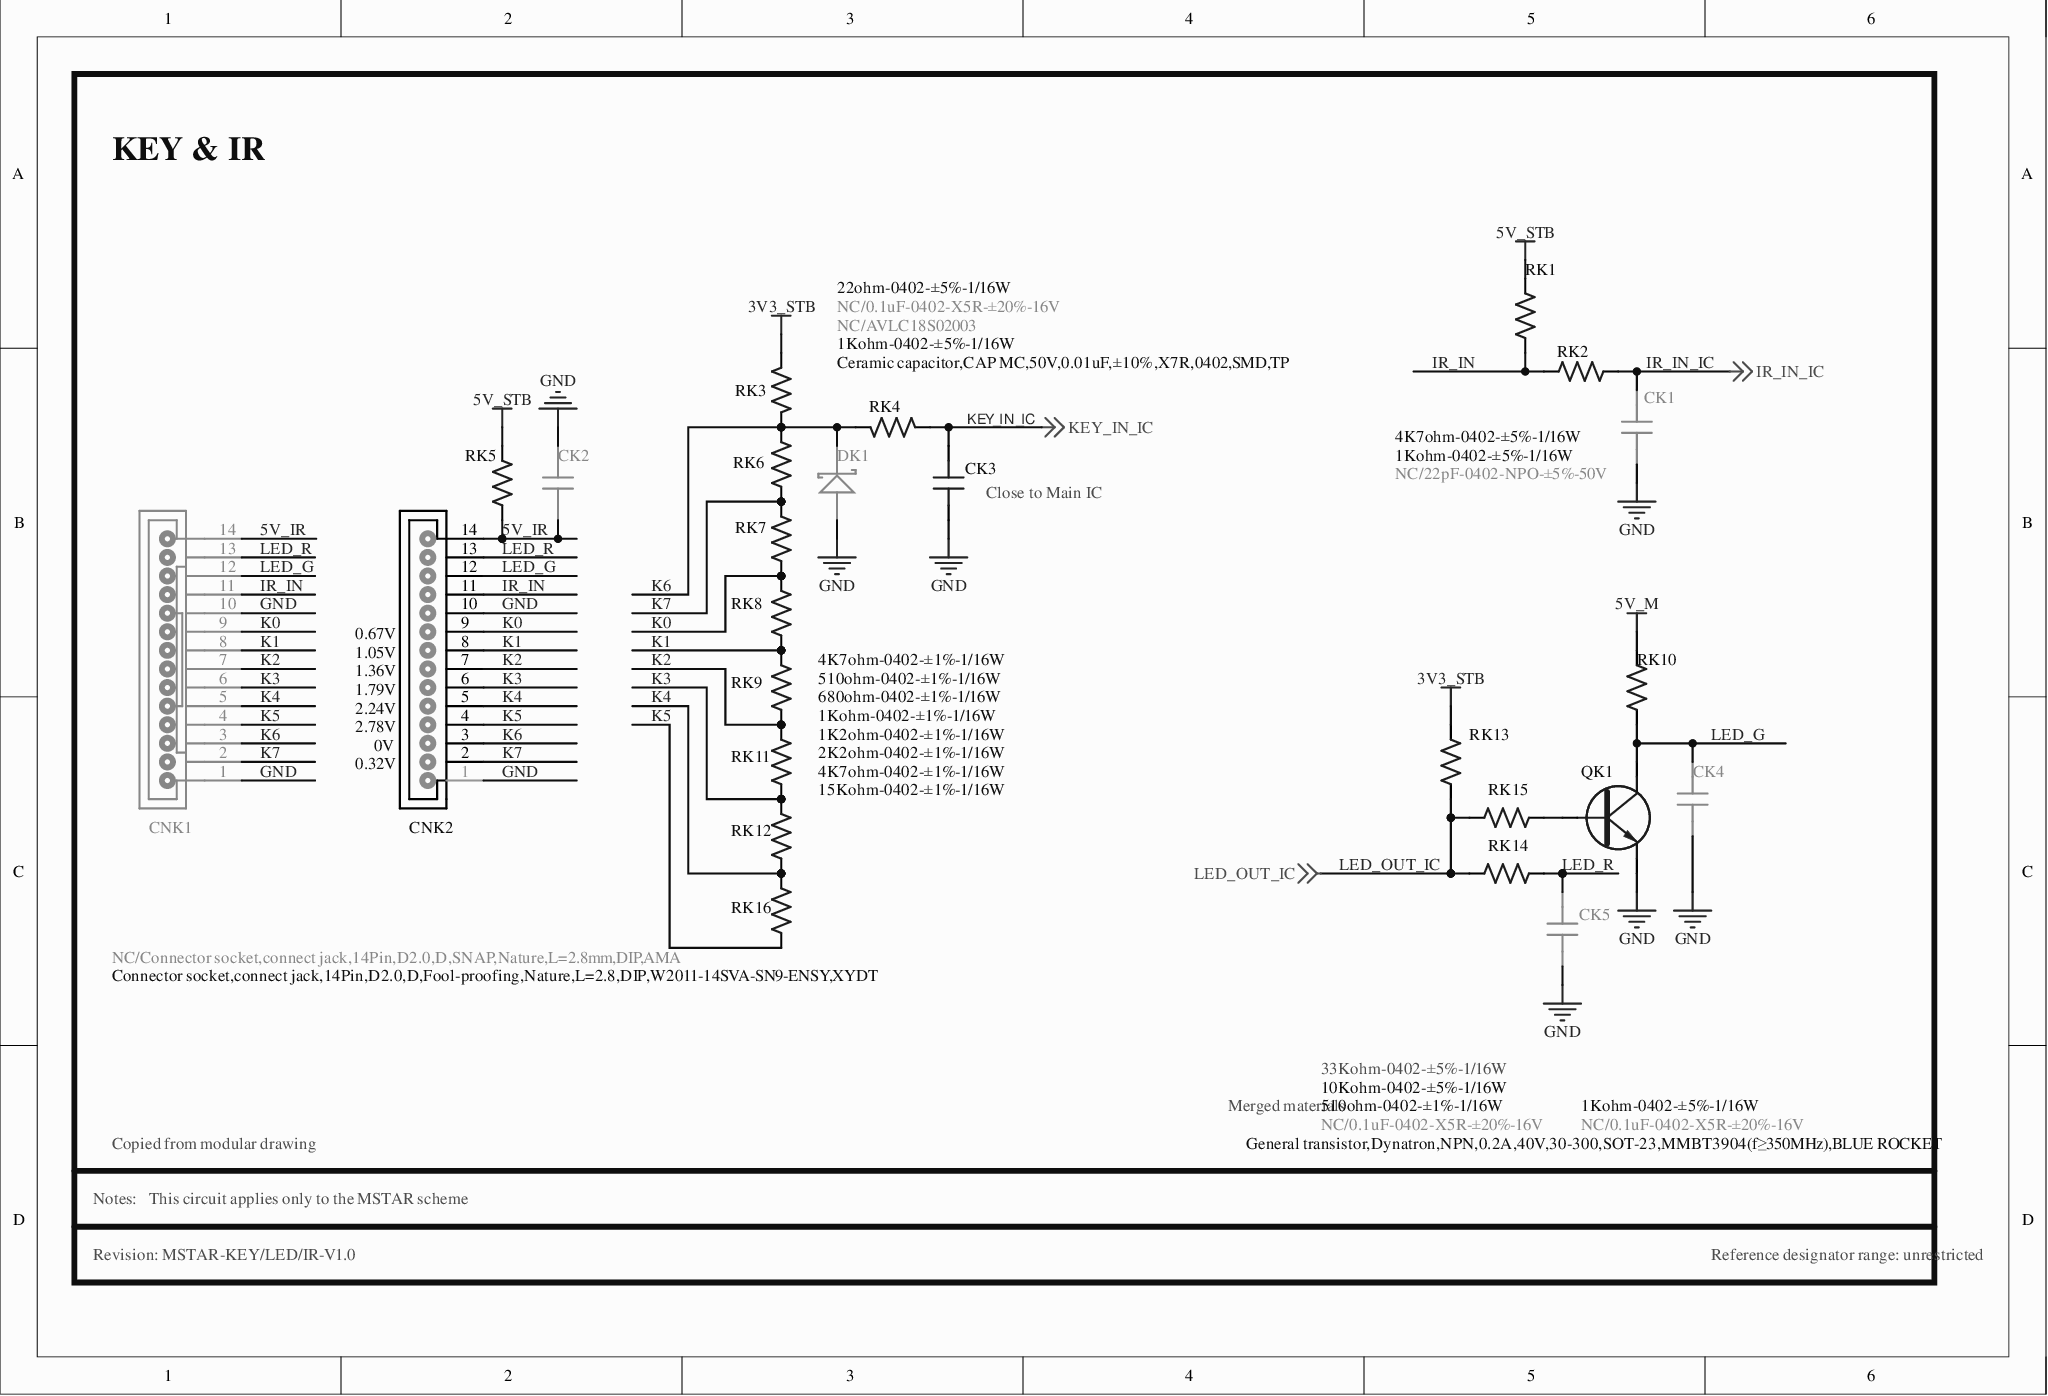
[diagram p0: MISC86372-10.SchDoc]
# Altium project MISC86372-32.PrjPCB (part 4 of 8)

## Sheet MISC86372-10.SchDoc
size 279 x 190 mm

### Parts
CK1  NC/22pF-0402-NPO-±5%-50V  [C0402]
CK2  NC/0.1uF-0402-X5R-±20%-16V  [C0402]
CK3  Ceramic capacitor,CAP MC,50V,0.01uF,±10%,X7R,0402,SMD,TP  [C0402]
CK4  NC/0.1uF-0402-X5R-±20%-16V  [C0402]
CK5  NC/0.1uF-0402-X5R-±20%-16V  [C0402]
CNK1  NC/Connector socket,connect jack,14Pin,D2.0,D,SNAP,Nature,L=2.8mm,DIP,AMA  [SIP14/2.0D-5]
CNK2  Connector socket,connect jack,14Pin,D2.0,D,Fool-proofing,Nature,L=2.8,DIP,W2011-14SVA-SN9-ENSY,XYDT  [SIP14/2.0D-1]
DK1  NC/AVLC18S02003  [DIODE-S0402]
QK1  General transistor,Dynatron,NPN,0.2A,40V,30-300,SOT-23,MMBT3904(f≥350MHz),BLUE ROCKET  [SOT-23]
RK1  4K7ohm-0402-±5%-1/16W  [R0402]
RK2  1Kohm-0402-±5%-1/16W  [R0402]
RK3  4K7ohm-0402-±1%-1/16W  [R0402]
RK4  1Kohm-0402-±5%-1/16W  [R0402]
RK5  22ohm-0402-±5%-1/16W  [R0402]
RK6  510ohm-0402-±1%-1/16W  [R0402]
RK7  680ohm-0402-±1%-1/16W  [R0402]
RK8  1Kohm-0402-±1%-1/16W  [R0402]
RK9  1K2ohm-0402-±1%-1/16W  [R0402]
RK10  1Kohm-0402-±5%-1/16W  [R0402]
RK11  2K2ohm-0402-±1%-1/16W  [R0402]
RK12  4K7ohm-0402-±1%-1/16W  [R0402]
RK13  33Kohm-0402-±5%-1/16W  [R0402]
RK14  510ohm-0402-±1%-1/16W  [R0402]
RK15  10Kohm-0402-±5%-1/16W  [R0402]
RK16  15Kohm-0402-±1%-1/16W  [R0402]

### Nets
3V3_STB: RK3.2 RK13.2
5V_M: RK10.2
5V_STB: RK1.2 RK5.1
GND: CK1.1 CK2.1 CK3.1 CK4.2 CK5.2 CNK1.1 CNK1.10 CNK2.1 CNK2.10 DK1.A QK1.E
5V_IR: CK2.2 CNK1.14 CNK2.14 RK5.2
IR_IN: CNK1.11 CNK2.11 RK1.1 RK2.1
IR_IN_IC: CK1.2 RK2.2 ; off-sheet IR_IN_IC
K0: CNK1.9 CNK2.9 RK7.1 RK8.2
K1: CNK1.8 CNK2.8 RK8.1 RK9.2
K2: CNK1.7 CNK2.7 RK9.1 RK11.2
K3: CNK1.6 CNK2.6 RK11.1 RK12.2
K4: CNK1.5 CNK2.5 RK12.1 RK16.2
K5: CNK1.4 CNK2.4 RK16.1
K6: CNK1.3 CNK2.3 DK1.K RK3.1 RK4.2 RK6.2
K7: CNK1.2 CNK2.2 RK6.1 RK7.2
KEY_IN_IC: CK3.2 RK4.1 ; off-sheet KEY_IN_IC
LED_G: CK4.1 CNK1.12 CNK2.12 QK1.C RK10.1
LED_OUT_IC: RK13.1 RK14.2 RK15.2 ; off-sheet LED_OUT_IC
LED_R: CK5.1 CNK1.13 CNK2.13 RK14.1
NetQK1_B: QK1.B RK15.1

### Notes on the sheet
- KEY & IR
- (near CK3) Close to Main IC
- (near CNK2) 0.67V
- (near CNK2) 1.05V
- (near CNK2) 1.36V
- (near CNK2) 1.79V
- (near CNK2) 2.24V
- (near CNK2) 2.78V
- (near CNK2) 0.32V
- (near CNK2) 0V
- Copied from modular drawing
- Merged materials
- Notes:
- This circuit applies only to the MSTAR scheme
- Revision: MSTAR-KEY/LED/IR-V1.0
- Reference designator range: unrestricted

### Library data of the parts
CK1 = 22pF-0402-NPO-±5%-50V-D
CK2 CK4 CK5 = 0.1uF-0402-X5R-±20%-16V-D
CK3 = 004.003.0000506-D: Ceramic capacitor,CAP MC,50V,0.01uF,±10%,X7R,0402,SMD,TP-D
CNK1 = 14PIN-2.0-D-H-G-带扣-J-DHMI
CNK2 = 14PIN-2.0-D-H-G-DHMI
DK1 = AVLC18S02003-D
QK1 = LMBT3904LT1G-D-NPN: Q-NPN-#-#-#
RK1 = 4K7ohm-0402-±5%-1/16W-D
RK2 RK4 RK10 = 1Kohm-0402-±5%-1/16W-D
RK3 RK12 = 4K7ohm-0402-±1%-1/16W-D
RK5 = 22ohm-0402-±5%-1/16W-D
RK6 RK14 = 510ohm-0402-±5%-1/16W-D
RK7 = 680ohm-0402-±1%-1/16W-D
RK8 = 1Kohm-0402-±1%-1/16W-D
RK9 = 1K2ohm-0402-±1%-1/16W-D
RK11 = 2K2ohm-0402-±1%-1/16W-D
RK13 = 33Kohm-0402-±5%-1/16W-D
RK15 = 10Kohm-0402-±5%-1/16W-D
RK16 = 15Kohm-0402-±1%-1/16W-D

## Sheet MISC86372-11.SchDoc
size 215 x 228 mm
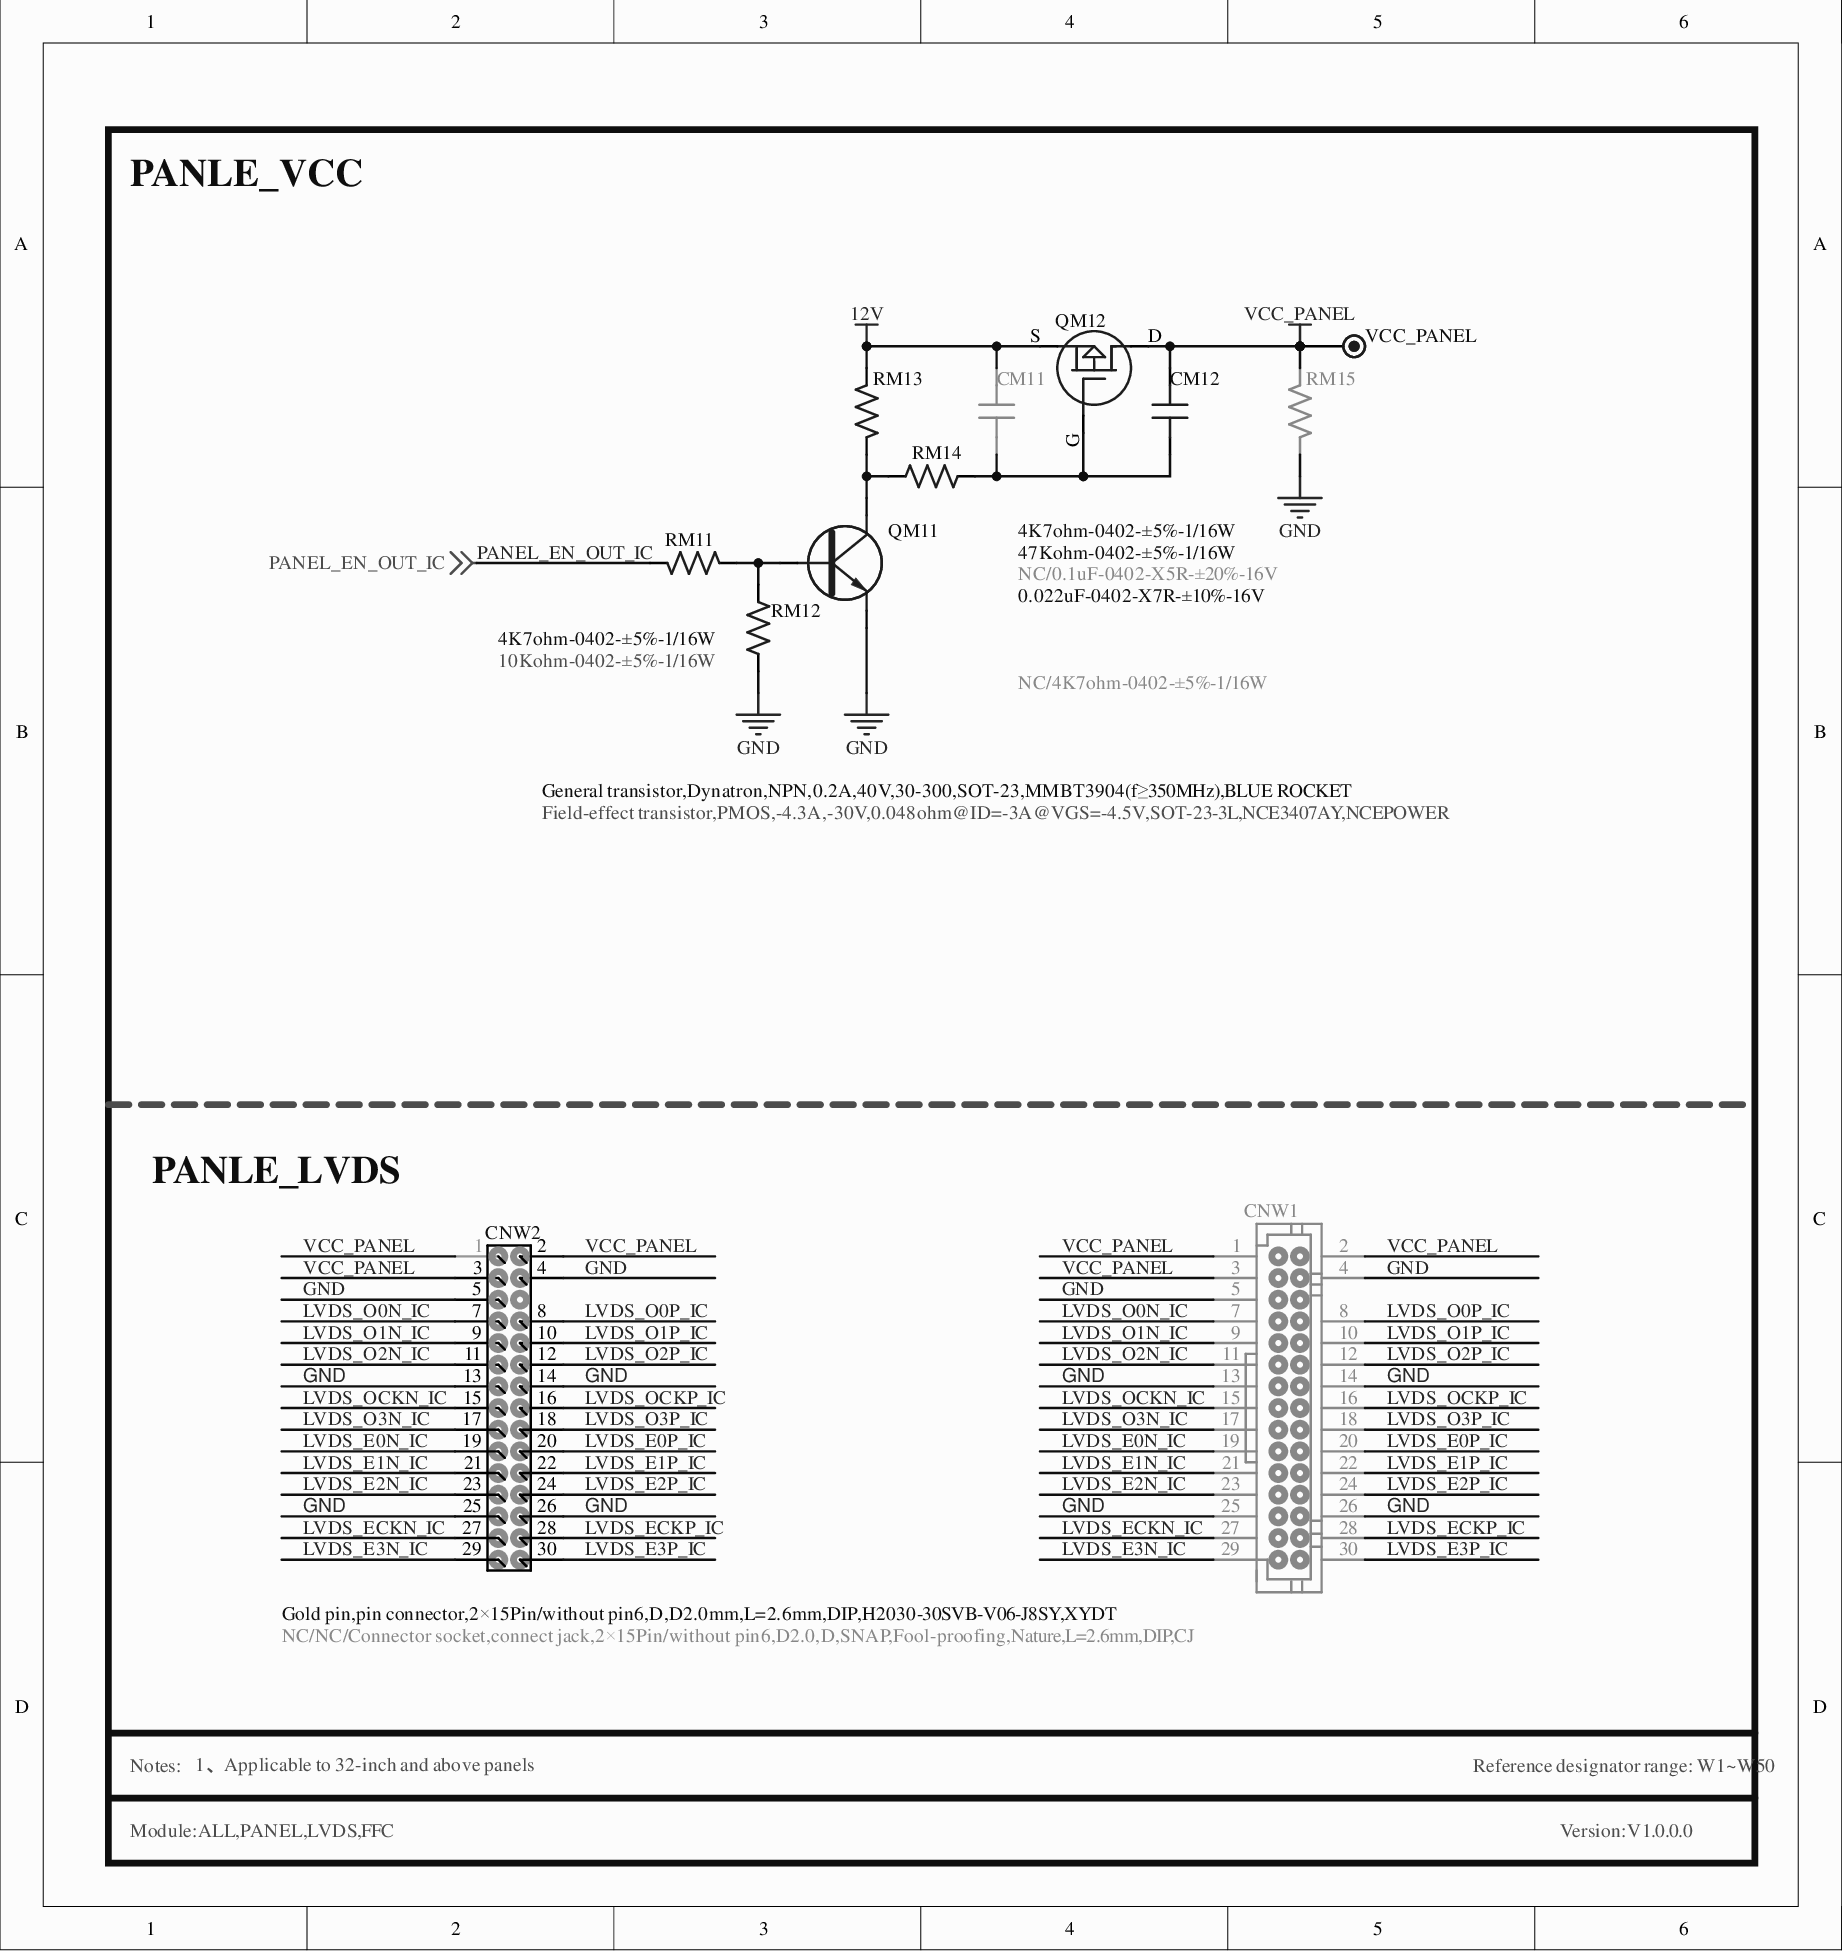
[diagram p1: MISC86372-11.SchDoc]

### Parts
CM11  NC/0.1uF-0402-X5R-±20%-16V  [C0402]
CM12  0.022uF-0402-X7R-±10%-16V  [C0402]
CNW1  NC/NC/Connector socket,connect jack,2×15Pin/without pin6,D2.0,D,SNAP,Fool-proofing,Nature,L=2.6mm,DIP,CJ  [SIP2*15/2.0D-11]
CNW2  Gold pin,pin connector,2×15Pin/without pin6,D,D2.0mm,L=2.6mm,DIP,H2030-30SVB-V06-J8SY,XYDT  [SIP2*15/2.0D-2]
QM11  General transistor,Dynatron,NPN,0.2A,40V,30-300,SOT-23,MMBT3904(f≥350MHz),BLUE ROCKET  [SOT-23]
QM12  Field-effect transistor,PMOS,-4.3A,-30V,0.048ohm@ID=-3A@VGS=-4.5V,SOT-23-3L,NCE3407AY,NCEPOWER  [SOT-23-1]
RM11  4K7ohm-0402-±5%-1/16W  [R0402]
RM12  10Kohm-0402-±5%-1/16W  [R0402]
RM13  4K7ohm-0402-±5%-1/16W  [R0402]
RM14  47Kohm-0402-±5%-1/16W  [R0402]
RM15  NC/4K7ohm-0402-±5%-1/16W  [R0402]
VCC_PANEL  TEST  [TP]  (value not drawn)

### Nets
12V: CM11.2 QM12.S RM13.1
GND: CNW1.4 CNW1.5 CNW1.13 CNW1.14 CNW1.25 CNW1.26 CNW2.4 CNW2.5 CNW2.13 CNW2.14 CNW2.25 CNW2.26 QM11.E RM12.2 RM15.2
VCC_PANEL: CM12.1 CNW1.1 CNW1.2 CNW1.3 CNW2.1 CNW2.2 CNW2.3 QM12.D RM15.1 VCC_PANEL.1
LVDS_E0N_IC: CNW1.19 CNW2.19
LVDS_E0P_IC: CNW1.20 CNW2.20
LVDS_E1N_IC: CNW1.21 CNW2.21
LVDS_E1P_IC: CNW1.22 CNW2.22
LVDS_E2N_IC: CNW1.23 CNW2.23
LVDS_E2P_IC: CNW1.24 CNW2.24
LVDS_E3N_IC: CNW1.29 CNW2.29
LVDS_E3P_IC: CNW1.30 CNW2.30
LVDS_ECKN_IC: CNW1.27 CNW2.27
LVDS_ECKP_IC: CNW1.28 CNW2.28
LVDS_O0N_IC: CNW1.7 CNW2.7
LVDS_O0P_IC: CNW1.8 CNW2.8
LVDS_O1N_IC: CNW1.9 CNW2.9
LVDS_O1P_IC: CNW1.10 CNW2.10
LVDS_O2N_IC: CNW1.11 CNW2.11
LVDS_O2P_IC: CNW1.12 CNW2.12
LVDS_O3N_IC: CNW1.17 CNW2.17
LVDS_O3P_IC: CNW1.18 CNW2.18
LVDS_OCKN_IC: CNW1.15 CNW2.15
LVDS_OCKP_IC: CNW1.16 CNW2.16
PANEL_EN_OUT_IC: RM11.1 ; off-sheet PANEL_EN_OUT_IC
NetCM11_1: CM11.1 CM12.2 QM12.G RM14.2
NetQM11_B: QM11.B RM11.2 RM12.1
NetQM11_C: QM11.C RM13.2 RM14.1

### Notes on the sheet
- PANLE_VCC
- PANLE_LVDS
- Notes:
- 1、 Applicable to 32-inch and above panels
- Reference designator range: W1~W50
- Module:ALL,PANEL,LVDS,FFC
- Version:V1.0.0.0

### Library data of the parts
CM11 = 0.1uF-0402-X5R-±20%-16V-D
CM12 = 0.022uF-0402-X7R-±10%-16V-D
CNW1 = 连接插座,connect jack,2×15Pin/without pin6,D2.0,D,SNAP,Fool-proofing,Nature,L=2.6mm,DIP,CJ: CN-latched
CNW2 = 2×15PIN-2.0-D-H-M(脚长=2.6mm)(缺6PIN)-LK-DHMI: CN-straight gold pin
QM11 = LMBT3904LT1G-D-NPN: Q-NPN-#-#-#
QM12 = WPM3407C-3/TR-D
RM11 RM13 RM15 = 4K7ohm-0402-±5%-1/16W-D
RM12 = 10Kohm-0402-±5%-1/16W-D
RM14 = 47Kohm-0402-±5%-1/16W-D

## Sheet MISC86372-12.SchDoc
size 444 x 355 mm
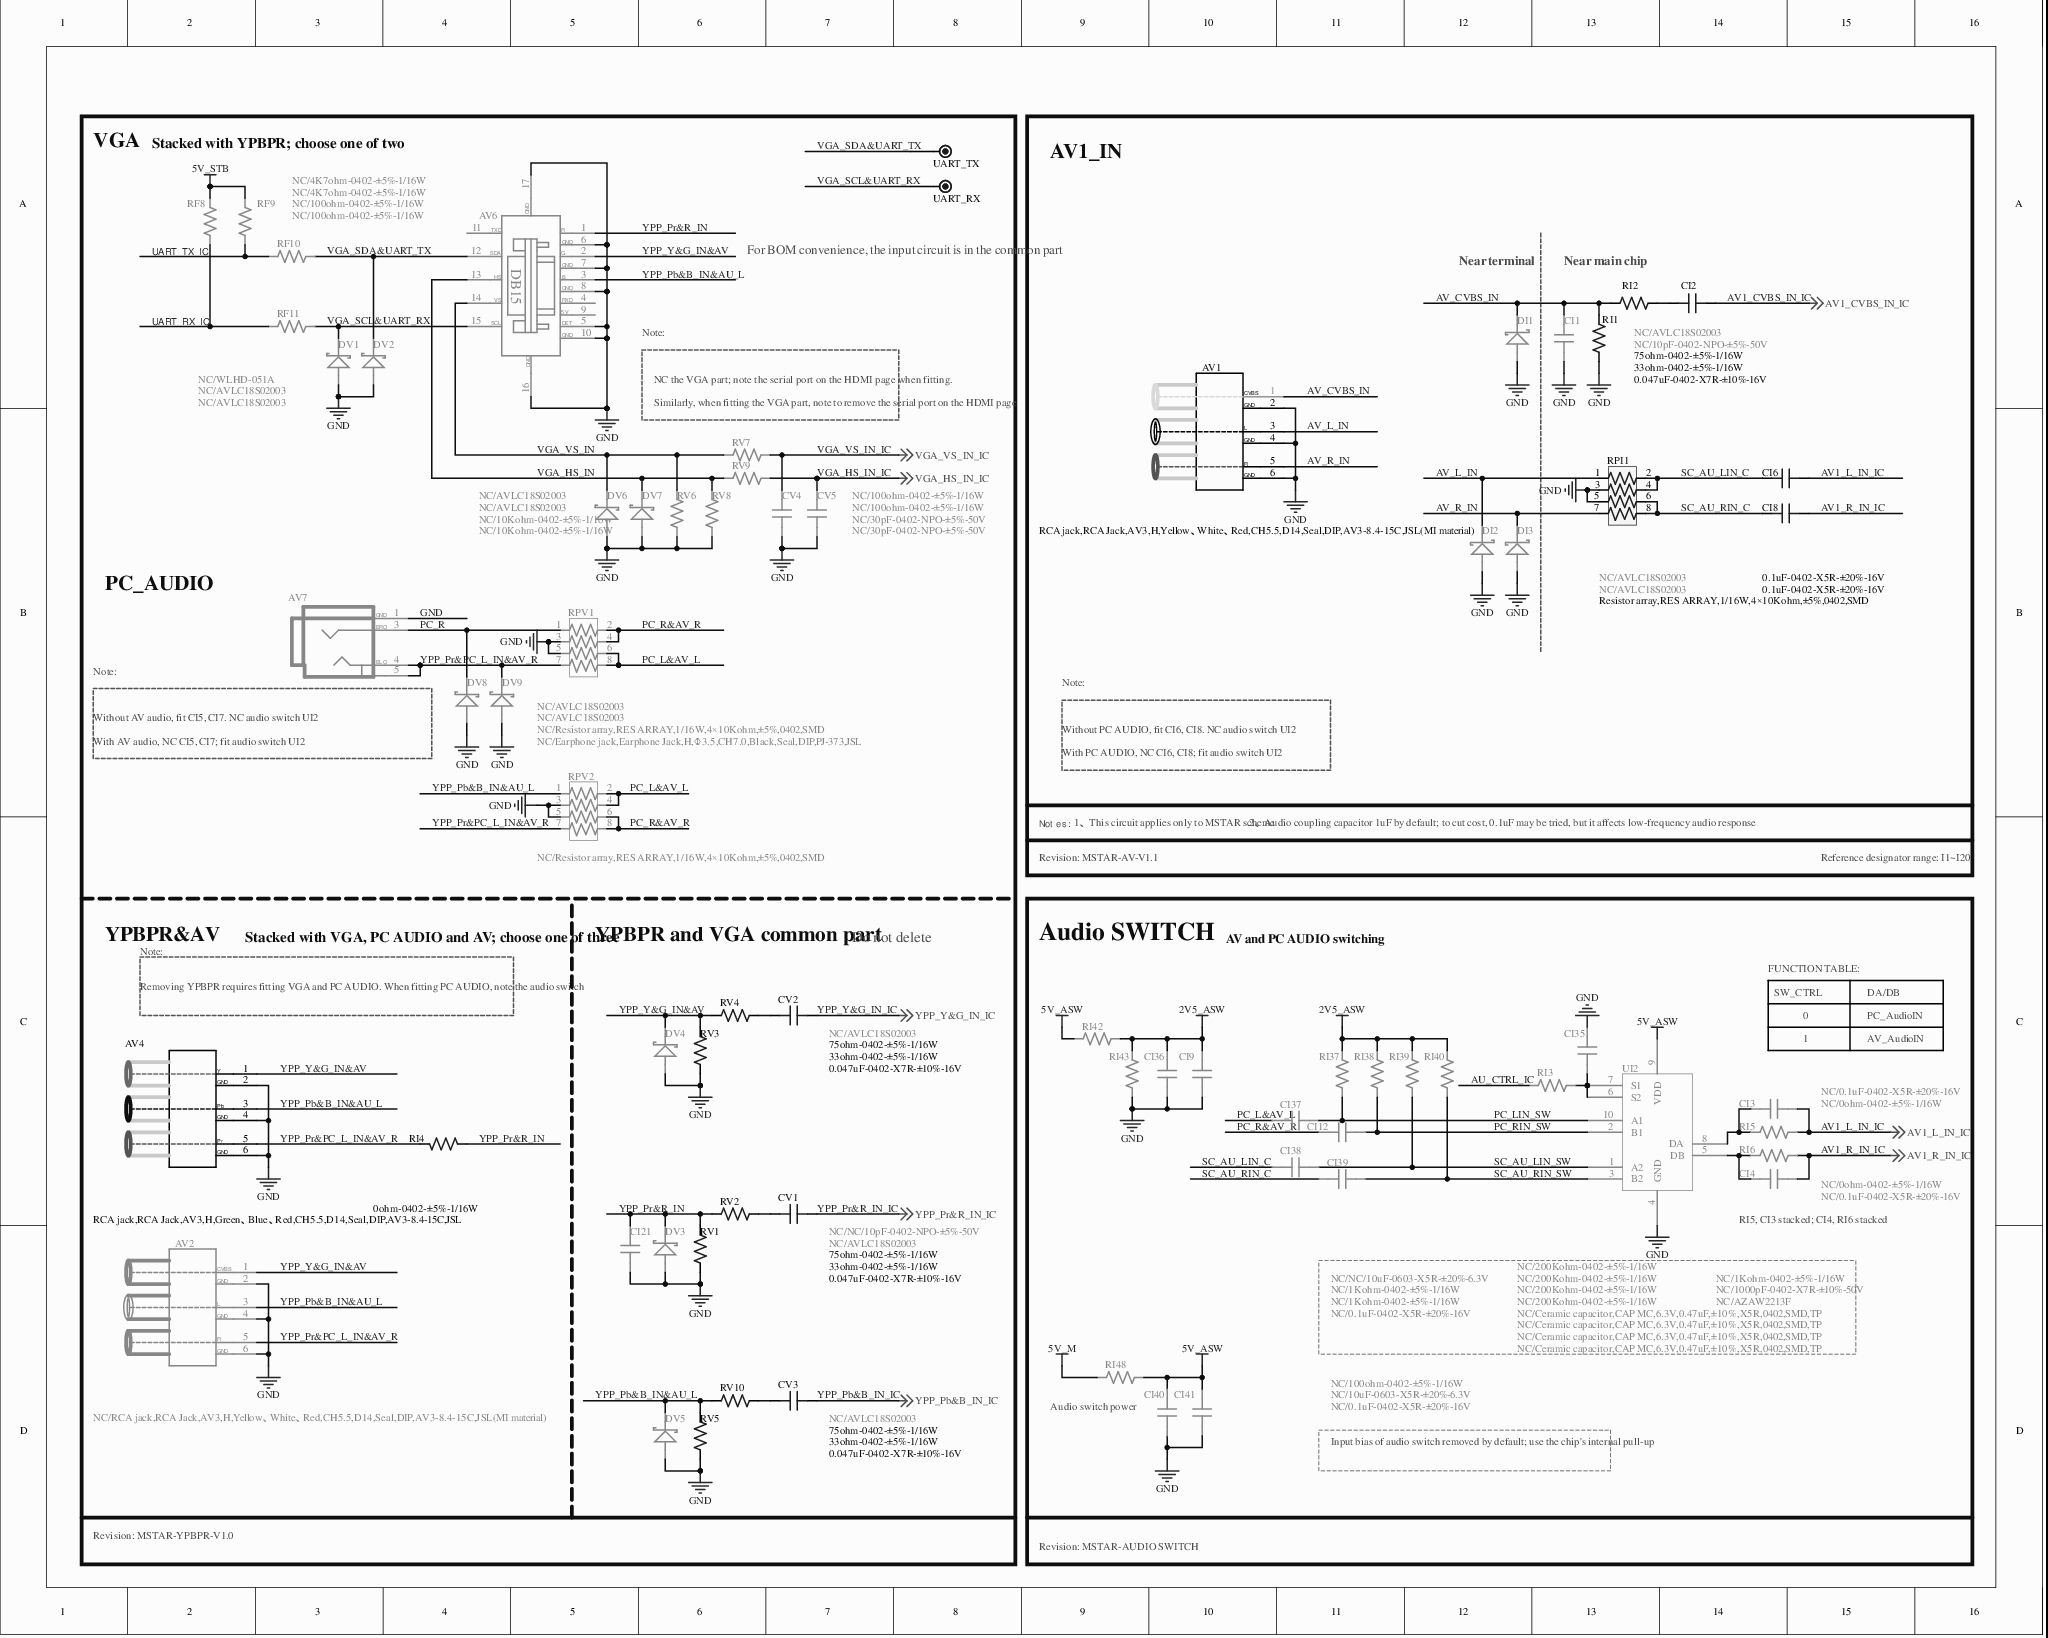
[diagram p2: MISC86372-12.SchDoc]

### Parts
AV1  RCA jack,RCA Jack,AV3,H,Yellow、White、Red,CH5.5,D14,Seal,DIP,AV3-8.4-15C,JSL(MI material)  [AV3-H14-15]
AV2  NC/RCA jack,RCA Jack,AV3,H,Yellow、White、Red,CH5.5,D14,Seal,DIP,AV3-8.4-15C,JSL(MI material)  [AV3-H14-15]
AV4  RCA jack,RCA Jack,AV3,H,Green、Blue、Red,CH5.5,D14,Seal,DIP,AV3-8.4-15C,JSL  [AV3-H14-15]
AV6  NC/WLHD-051A  [DB15-HF-1]
AV7  NC/Earphone jack,Earphone Jack,H,Φ3.5,CH7.0,Black,Seal,DIP,PJ-373,JSL  [PHONE-HD-41]
CI1  NC/10pF-0402-NPO-±5%-50V  [C0402]
CI2  0.047uF-0402-X7R-±10%-16V  [C0402]
CI3  NC/0.1uF-0402-X5R-±20%-16V  [C0402]
CI4  NC/0.1uF-0402-X5R-±20%-16V  [C0402]
CI6  0.1uF-0402-X5R-±20%-16V  [C0402]
CI8  0.1uF-0402-X5R-±20%-16V  [C0402]
CI9  NC/NC/10uF-0603-X5R-±20%-6.3V  [C0603]
CI12  NC/Ceramic capacitor,CAP MC,6.3V,0.47uF,±10%,X5R,0402,SMD,TP  [C0402]
CI21  NC/NC/10pF-0402-NPO-±5%-50V  [C0402]
CI35  NC/1000pF-0402-X7R-±10%-50V  [C0402]
CI36  NC/0.1uF-0402-X5R-±20%-16V  [C0402]
CI37  NC/Ceramic capacitor,CAP MC,6.3V,0.47uF,±10%,X5R,0402,SMD,TP  [C0402]
CI38  NC/Ceramic capacitor,CAP MC,6.3V,0.47uF,±10%,X5R,0402,SMD,TP  [C0402]
CI39  NC/Ceramic capacitor,CAP MC,6.3V,0.47uF,±10%,X5R,0402,SMD,TP  [C0402]
CI40  NC/10uF-0603-X5R-±20%-6.3V  [C0603]
CI41  NC/0.1uF-0402-X5R-±20%-16V  [C0402]
CV1  0.047uF-0402-X7R-±10%-16V  [C0402]
CV2  0.047uF-0402-X7R-±10%-16V  [C0402]
CV3  0.047uF-0402-X7R-±10%-16V  [C0402]
CV4  NC/30pF-0402-NPO-±5%-50V  [C0402]
CV5  NC/30pF-0402-NPO-±5%-50V  [C0402]
DI1  NC/AVLC18S02003  [DIODE-S0402]
DI2  NC/AVLC18S02003  [DIODE-S0402]
DI3  NC/AVLC18S02003  [DIODE-S0402]
DV1  NC/AVLC18S02003  [DIODE-S0402]
DV2  NC/AVLC18S02003  [DIODE-S0402]
DV3  NC/AVLC18S02003  [DIODE-S0402]
DV4  NC/AVLC18S02003  [DIODE-S0402]
DV5  NC/AVLC18S02003  [DIODE-S0402]
DV6  NC/AVLC18S02003  [DIODE-S0402]
DV7  NC/AVLC18S02003  [DIODE-S0402]
DV8  NC/AVLC18S02003  [DIODE-S0402]
DV9  NC/AVLC18S02003  [DIODE-S0402]
RF8  NC/4K7ohm-0402-±5%-1/16W  [R0402]
RF9  NC/4K7ohm-0402-±5%-1/16W  [R0402]
RF10  NC/100ohm-0402-±5%-1/16W  [R0402]
RF11  NC/100ohm-0402-±5%-1/16W  [R0402]
RI1  75ohm-0402-±5%-1/16W  [R0402]
RI2  33ohm-0402-±5%-1/16W  [R0402]
RI3  NC/1Kohm-0402-±5%-1/16W  [R0402]
RI4  0ohm-0402-±5%-1/16W  [R0402]
RI5  NC/0ohm-0402-±5%-1/16W  [R0402]
RI6  NC/0ohm-0402-±5%-1/16W  [R0402]
RI37  NC/200Kohm-0402-±5%-1/16W  [R0402]
RI38  NC/200Kohm-0402-±5%-1/16W  [R0402]
RI39  NC/200Kohm-0402-±5%-1/16W  [R0402]
RI40  NC/200Kohm-0402-±5%-1/16W  [R0402]
RI42  NC/1Kohm-0402-±5%-1/16W  [R0402]
RI43  NC/1Kohm-0402-±5%-1/16W  [R0402]
RI48  NC/100ohm-0402-±5%-1/16W  [R0402]
RPI1  Resistor array,RES ARRAY,1/16W,4×10Kohm,±5%,0402,SMD  [RA0402]
RPV1  NC/Resistor array,RES ARRAY,1/16W,4×10Kohm,±5%,0402,SMD  [RA0402]
RPV2  NC/Resistor array,RES ARRAY,1/16W,4×10Kohm,±5%,0402,SMD  [RA0402]
RV1  75ohm-0402-±5%-1/16W  [R0402]
RV2  33ohm-0402-±5%-1/16W  [R0402]
RV3  75ohm-0402-±5%-1/16W  [R0402]
RV4  33ohm-0402-±5%-1/16W  [R0402]
RV5  75ohm-0402-±5%-1/16W  [R0402]
RV6  NC/10Kohm-0402-±5%-1/16W  [R0402]
RV7  NC/100ohm-0402-±5%-1/16W  [R0402]
RV8  NC/10Kohm-0402-±5%-1/16W  [R0402]
RV9  NC/100ohm-0402-±5%-1/16W  [R0402]
RV10  33ohm-0402-±5%-1/16W  [R0402]
UART_RX  DM0  [TP]  (value not drawn)
UART_TX  DM0  [TP]  (value not drawn)
UI2  NC/AZAW2213F  [QFN10/0.4]

### Blocks framed on the sheet
AV1_IN: AV1 CI1 CI2 CI6 CI8 DI1-DI3 RI1 RI2 RPI1
Audio SWITCH: CI3 CI4 CI9 CI12 CI35-CI41 RI3 RI5 RI6 RI37-RI40 RI42 RI43 RI48 UI2

### Nets
2V5_ASW: CI9.2 CI36.2 RI37.2 RI38.2 RI39.2 RI40.2 RI42.2 RI43.2
5V_ASW: CI40.2 CI41.2 RI42.1 RI48.2 UI2.9(VDD)
5V_M: RI48.1
5V_STB: RF8.2 RF9.2
GND: AV1.2(GND) AV1.4 AV1.6 AV2.2(GND) AV2.4 AV2.6 AV4.2(CVBS) AV4.4(Rin) AV4.6(Lin) AV6.5 AV6.6(GND) AV6.7(GND) AV6.8(GND) AV6.10(GND) AV6.16(Shell) AV6.17(Shell) AV7.1 CI1.2 CI9.1 CI21.2 CI35.2 CI36.1 CI40.1 CI41.1 CV4.1 CV5.1 DI1.A DI2.A DI3.A DV1.A DV2.A DV3.A DV4.A DV5.A DV6.A DV7.A DV8.A DV9.A RI1.1 RI43.1 RPI1.3 RPI1.5 RPV1.3 RPV1.5 RPV2.3 RPV2.5 RV1.1 RV3.1 RV5.1 RV6.1 RV8.1 UI2.4(GND)
AU_CTRL_IC: RI3.1
AV1_CVBS_IN_IC: CI2.2 ; off-sheet AV1_CVBS_IN_IC
AV1_L_IN_IC: CI3.1 CI6.1 RI5.2 ; off-sheet AV1_L_IN_IC
AV1_R_IN_IC: CI4.1 CI8.1 RI6.2 ; off-sheet AV1_R_IN_IC
AV_CVBS_IN: AV1.1(R) CI1.1 DI1.K RI1.2 RI2.2
AV_L_IN: AV1.3 DI2.K RPI1.1
AV_R_IN: AV1.5 DI3.K RPI1.7
PC_L&AV_L: CI37.2 RPV1.6 RPV1.8 RPV2.2 RPV2.4
PC_LIN_SW: CI37.1 RI37.1 UI2.10(A1)
PC_R: AV7.3 DV8.K RPV1.1
PC_R&AV_R: CI12.2 RPV1.2 RPV1.4 RPV2.6 RPV2.8
PC_RIN_SW: CI12.1 RI38.1 UI2.2(B1)
SC_AU_LIN_C: CI6.2 CI38.2 RPI1.2 RPI1.4
SC_AU_LIN_SW: CI38.1 RI39.1 UI2.1(A2)
SC_AU_RIN_C: CI8.2 CI39.2 RPI1.6 RPI1.8
SC_AU_RIN_SW: CI39.1 RI40.1 UI2.3(B2)
UART_RX_IC: RF8.1 RF11.1
UART_TX_IC: RF9.1 RF10.1
VGA_HS_IN: AV6.13(HS) DV7.K RV8.2 RV9.1
VGA_HS_IN_IC: CV5.2 RV9.2 ; off-sheet VGA_HS_IN_IC
VGA_SCL&UART_RX: AV6.15(SCL) DV1.K RF11.2 UART_RX.1
VGA_SDA&UART_TX: AV6.12(SDA) DV2.K RF10.2 UART_TX.1
VGA_VS_IN: AV6.14(VS) DV6.K RV6.2 RV7.1
VGA_VS_IN_IC: CV4.2 RV7.2 ; off-sheet VGA_VS_IN_IC
YPP_Pb&B_IN&AU_L: AV2.3 AV4.3(GND) AV6.3(B) DV5.K RPV2.1 RV5.2 RV10.1
YPP_Pb&B_IN_IC: CV3.2 ; off-sheet YPP_Pb&B_IN_IC
YPP_Pr&PC_L_IN&AV_R: AV2.5 AV4.5(GND) AV7.4 AV7.5 DV9.K RI4.2 RPV1.7 RPV2.7
YPP_Pr&R_IN: AV6.1(R) CI21.1 DV3.K RI4.1 RV1.2 RV2.1
YPP_Pr&R_IN_IC: CV1.2 ; off-sheet YPP_Pr&R_IN_IC
YPP_Y&G_IN&AV: AV2.1(R) AV4.1(GND) AV6.2(G) DV4.K RV3.2 RV4.1
YPP_Y&G_IN_IC: CV2.2 ; off-sheet YPP_Y&G_IN_IC
NetCI2_1: CI2.1 RI2.1
NetCI3_2: CI3.2 RI5.1 UI2.8(DA)
NetCI4_2: CI4.2 RI6.1 UI2.5(DB)
NetCI35_1: CI35.1 RI3.2 UI2.6(S2) UI2.7(S1)
NetCV1_1: CV1.1 RV2.2
NetCV2_1: CV2.1 RV4.2
NetCV3_1: CV3.1 RV10.2

Not connected (* = marked no-connect by the designer): AV6 4(NC)* 9(NC)* 11(NC)*

### Notes on the sheet
- VGA
- Stacked with YPBPR; choose one of two
- For BOM convenience, the input circuit is in the common part
- Near terminal
- Near main chip
- Note:
- NC the VGA part; note the serial port on the HDMI page when fitting.
- Similarly, when fitting the VGA part, note to remove the serial port on the HDMI page
- PC_AUDIO
- (near AV7) Without AV audio, fit CI5, CI7. NC audio switch UI2
- With AV audio, NC CI5, CI7; fit audio switch UI2
- Without PC AUDIO, fit CI6, CI8. NC audio switch UI2
- With PC AUDIO, NC CI6, CI8; fit audio switch UI2
- Notes:
- 1、 This circuit applies only to MSTAR scheme
- 2、 Audio coupling capacitor 1uF by default; to cut cost, 0.1uF may be tried, but it affects low-frequency audio response
- Revision: MSTAR-AV-V1.1
- Reference designator range: I1~I20
- YPBPR&AV
- Stacked with VGA, PC AUDIO and AV; choose one of three
- YPBPR and VGA common part
- Do not delete
- AV and PC AUDIO switching
- Removing YPBPR requires fitting VGA and PC AUDIO. When fitting PC AUDIO, note the audio switch
- FUNCTION TABLE:
- SW_CTRL
- DA/DB
- 0
- 1
- PC_AudioIN
- AV_AudioIN
- RI5, CI3 stacked; CI4, RI6 stacked
- Audio switch power
- Input bias of audio switch removed by default; use the chip's internal pull-up
- Revision: MSTAR-YPBPR-V1.0
- Revision: MSTAR-AUDIO SWITCH

### Library data of the parts
AV1 AV2 = RCA端子,RCA Jack,AV3,H,Yellow、White、Red,CH5.5,D14,Seal,DIP,RC075-F03L3BY-A,YUQIU-DLMI-AV: CN-AV-D14-#-#
AV4 = RCA端子,RCA Jack,AV3,H,Green、Blue、Red,CH5.5,D14,Seal,DIP,RC075-F03L3BY-B,YUQIU-DLMI-YPbPr: CN-YPbPr-D14-#-#
AV6 = WLHD-051A-DLMI-DB15: CN-DB15-horizontal-#-#-#
AV7 = 耳机端子,Earphone  Jack,H,Φ3.5,CH7.0,Black,Seal,SMD,PJ7723-F03L3BE-C,YUQIU-DLMI: CN-headphone
CI1 CI21 = 10pF-0402-NPO-±5%-50V-D
CI2 CV1-CV3 = 0.047uF-0402-X7R-±10%-16V-D
CI3 CI4 CI6 CI8 = 0.1uF-0402-Y5V-+80%-20%-16V-D
CI9 CI40 = 10uF-0603-X5R-±20%-6.3V-D
CI12 CI37-CI39 = 004.003.0000361-D: Ceramic capacitor,CAP MC,6.3V,0.47uF,±10%,X5R,0402,SMD,TP-D
CI35 = 1000pF-0402-X7R-±10%-50V-D
CI36 CI41 = 0.1uF-0402-X5R-±20%-16V-D
CV4 CV5 = 30pF-0402-NPO-±5%-50V-D
DI1-DI3 = AIES12U020R2-D
DV1-DV9 = AVLC18S02003-D
RF8 RF9 = 4K7ohm-0402-±5%-1/16W-D
RF10 RF11 RI48 RV7 RV9 = 100ohm-0402-±5%-1/16W-D
RI1 RV1 RV3 RV5 = 75ohm-0402-±5%-1/16W-D
RI2 RV2 RV4 RV10 = 33ohm-0402-±5%-1/16W-D
RI3 RI42 RI43 = 1Kohm-0402-±5%-1/16W-D
RI4 = 004.002.0000558-D: Thick-film resistor,RES,1/16W,0ohm,±5%,0402,SMD-D
RI5 RI6 = 0ohm-0402-±5%-1/16W-D
RI37-RI40 = 200Kohm-0402-±5%-1/16W-D
RPI1 RPV1 RPV2 = 4*100ohm-0402-±5%-1/16W-D
RV6 RV8 = 10Kohm-0402-±5%-1/16W-D
UART_RX UART_TX = TEST
UI2 = AZAW2213F-D